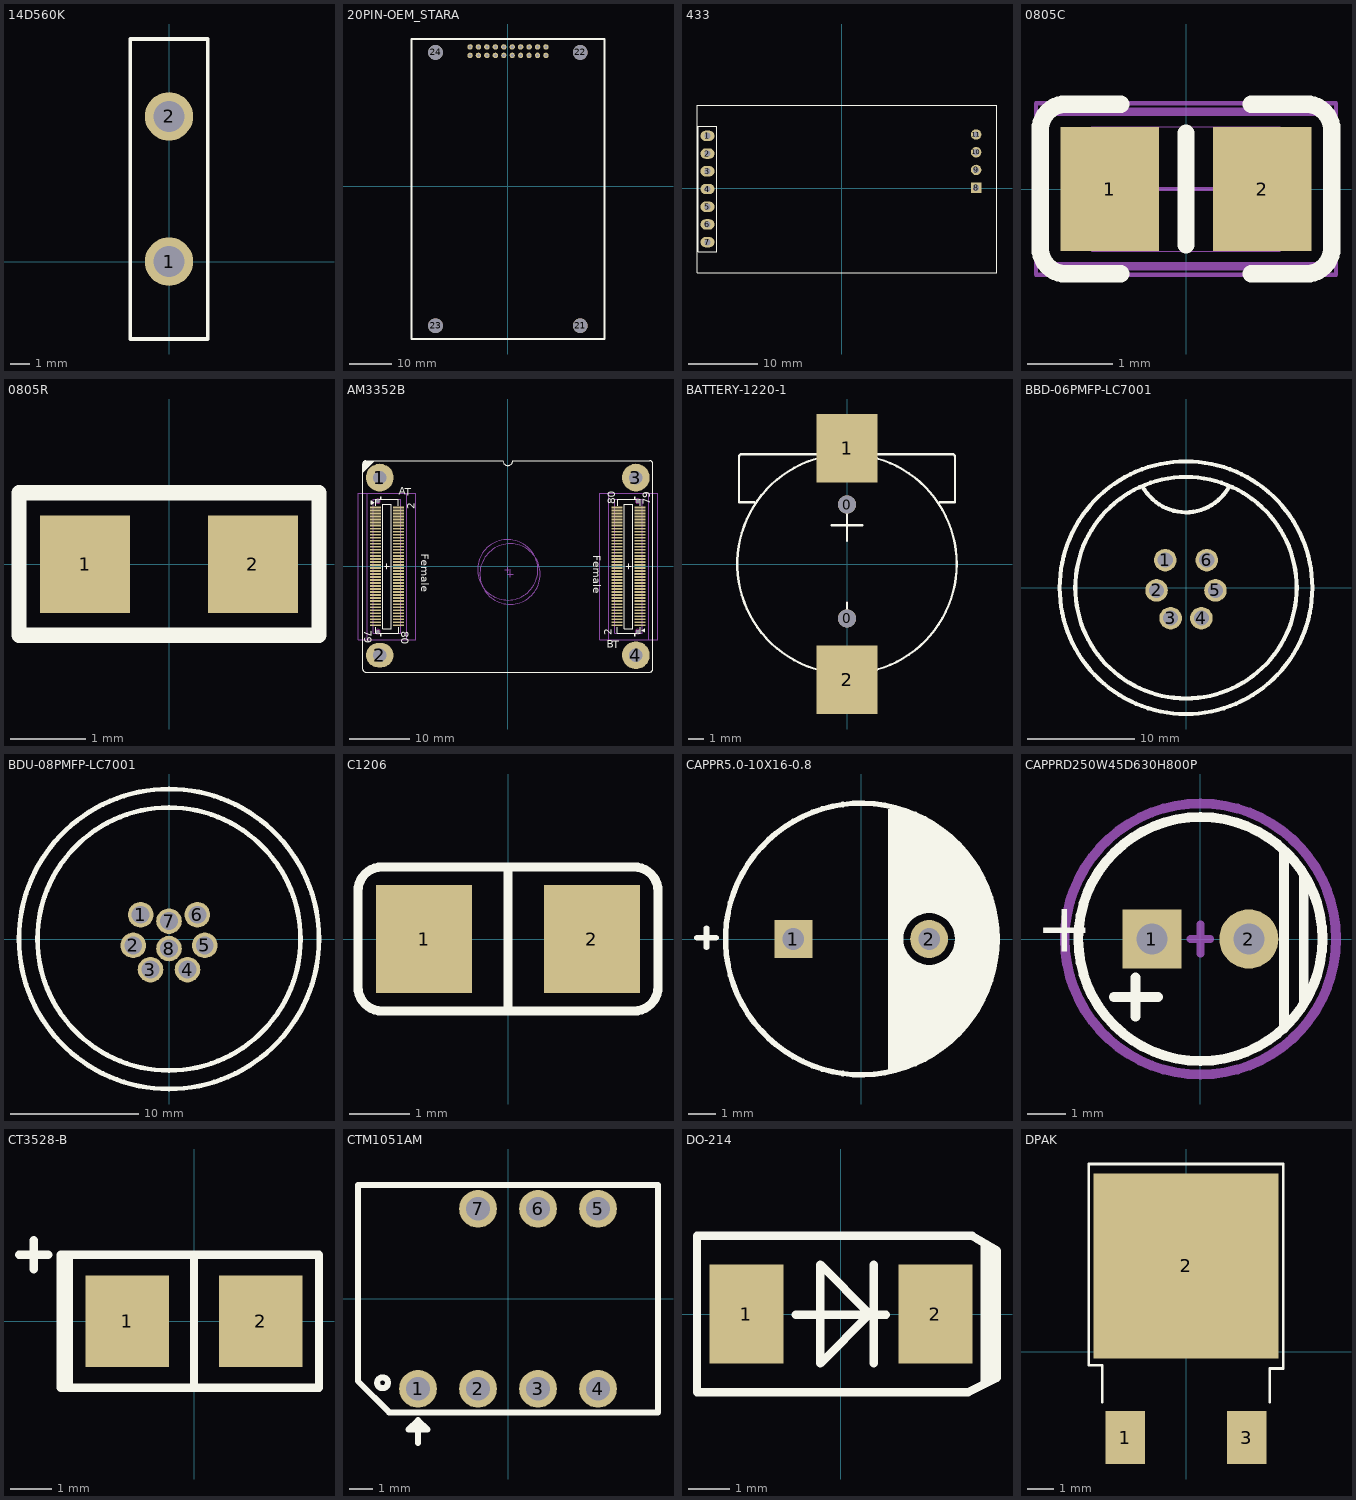
[diagram p0: the footprints below, top view; thin cyan lines are the x and y axes]
# Altium footprint library MISC82794-2.PcbLib: 41 footprints (part 1 of 3)
Each footprint in its own frame and in the unit in brackets; x right, y up, seen from the top. Pads: shape width x height; smd on the part's side, far side on the other; paste and mask are expansions set on the pad; w line width, h text height; cw(c..) or ccw(c..) is an arc to the next point about the centre after c.

## 14D560K [mm]
height 3.98
pads (2):
  round 2.5 hole 1.6: 1(0,0) 2(0,7.5)
Top Overlay:
  lines w0.2: -2,-4 -2,11.5 2,11.5 2,-4 -2,-4

## 20PIN-OEM_STARA [mm]
height 9.5
pads (24):
  round 1.3 hole 0.737: 1(-8.975,33.025) 2(-8.975,31.025) 3(-6.975,33.025) 4(-6.975,31.025) 5(-4.975,33.025) 6(-4.975,31.025) 7(-2.975,33.025) 8(-2.975,31.025) 9(-0.975,33.025) 11(1.025,33.025) 13(3.025,33.025) 15(5.025,33.025) 17(7.025,33.025) 19(9.025,33.025) 20(9.025,31.025)
  oval 1.2x1.3 hole 0.737: 10(-0.975,31.025) 12(1.025,31.025) 14(3.025,31.025) 16(5.025,31.025) 18(7.025,31.025)
  round 3.5 hole 3.5: 21(17.145,-33.025) 22(17.145,31.745) 23(-17.145,-33.025) 24(-17.145,31.745)
Top Overlay:
  lines w0.5: -22.805,-36.185 22.855,-36.185 22.855,34.915 -22.805,34.915 -22.805,-36.185

## 433 [mm]
pads (11):
  oval 2x1.5 hole 0.9: 1(-19.25,7.525) 2(-19.25,4.985) 3(-19.25,2.445) 4(-19.25,-0.095) 5(-19.25,-2.635) 6(-19.25,-5.175) 7(-19.25,-7.715)
  rect 1.5x1.5 hole 0.9: 8(19.25,0.095)
  round 1.5 hole 0.9: 9(19.25,2.635) 10(19.25,5.175) 11(19.25,7.715)
Top Overlay:
  lines w0.1: -20.75,-12.095 22.25,-12.095 22.25,11.905 -20.75,11.905 -20.75,-12.095
  lines w0.127: -20.55,-9.095 -20.55,8.905 -17.95,8.905 -17.95,-9.095 -20.55,-9.095

## 0805C [mm]
height 9.5
pads (2):
  rect 1.15x1.45 smd: 1(-0.889,0) 2(0.889,0)
Top Overlay:
  lines w0.2: 0,-0.65 0,0.65
  lines w0.203: -0.762,-0.991 -1.397,-0.991 cw(c-1.397,-0.686) -1.702,-0.686 -1.702,0.686 cw(c-1.397,0.686) -1.397,0.991 -0.762,0.991 ; 0.762,-0.991 1.397,-0.991 ccw(c1.397,-0.686) 1.702,-0.686 1.702,0.686 ccw(c1.397,0.686) 1.397,0.991 0.762,0.991
Mechanical 15:
  lines w0.1: -1.65,-0.9 -1.65,0.9 1.65,0.9 1.65,-0.9 -1.65,-0.9
  text "1" at -0.164,-0.45 h1.27
Mechanical 16:
  lines w0.001: -1.1,-0.725 -1.1,0.725 1.1,0.725 1.1,-0.725 -1.1,-0.725
  lines w0.05: -0.5,0 0.5,0 ; 0,-0.5 0,0.5 ; -1.75,-1 -1.75,1 1.75,1 1.75,-1 -1.75,-1
3D body: height 0.78, standoff 0, extent -1,-0.625 1,0.625

## 0805R [mm]
height 1.2
pads (2):
  rect 1.2x1.3 smd: 1(-1.118,0) 2(1.118,0)
Top Overlay:
  lines w0.203: -2,-0.95 -2,0.95 2,0.95 2,-0.95 -2,-0.95

## AM3352B [mm]
height 3.98
pads (172):
  round 0.6 hole 0.6 unplated mask+0.254: 0(-21.5,-10.8) 0(-21.5,-10.8) 0(-21.5,10.8) 0(-21.5,10.8) 0(21.5,-10.8) 0(21.5,-10.8) 0(21.5,10.8) 0(21.5,10.8)
  round 4.6 hole 2.2: 1(-21.2,14.7) 3(21.2,14.7) 4(21.2,-14.7)
  oval 4.6x4 hole 2.2: 2(-21.2,-14.7)
  rect 1.8x0.3 smd: A1(-21.9,9.75) A2(-18.1,9.75) A3(-21.9,9.25) A4(-18.1,9.25) A5(-21.9,8.75) A6(-18.1,8.75) A7(-21.9,8.25) A8(-18.1,8.25) A9(-21.9,7.75) A10(-18.1,7.75) A11(-21.9,7.25) A12(-18.1,7.25) A13(-21.9,6.75) A14(-18.1,6.75) A15(-21.9,6.25) A16(-18.1,6.25) A17(-21.9,5.75) A18(-18.1,5.75) A19(-21.9,5.25) A20(-18.1,5.25) A21(-21.9,4.75) A22(-18.1,4.75) A23(-21.9,4.25) A24(-18.1,4.25) A25(-21.9,3.75) A26(-18.1,3.75) A27(-21.9,3.25) A28(-18.1,3.25) A29(-21.9,2.75) A30(-18.1,2.75) A31(-21.9,2.25) A32(-18.1,2.25) A33(-21.9,1.75) A34(-18.1,1.75) A35(-21.9,1.25) A36(-18.1,1.25) A37(-21.9,0.75) A38(-18.1,0.75) A39(-21.9,0.25) A40(-18.1,0.25) A41(-21.9,-0.25) A42(-18.1,-0.25) A43(-21.9,-0.75) A44(-18.1,-0.75) A45(-21.9,-1.25) A46(-18.1,-1.25) A47(-21.9,-1.75) A48(-18.1,-1.75) A49(-21.9,-2.25) A50(-18.1,-2.25) A51(-21.9,-2.75) A52(-18.1,-2.75) A53(-21.9,-3.25) A54(-18.1,-3.25) A55(-21.9,-3.75) A56(-18.1,-3.75) A57(-21.9,-4.25) A58(-18.1,-4.25) A59(-21.9,-4.75) A60(-18.1,-4.75) A61(-21.9,-5.25) A62(-18.1,-5.25) A63(-21.9,-5.75) A64(-18.1,-5.75) A65(-21.9,-6.25) A66(-18.1,-6.25) A67(-21.9,-6.75) A68(-18.1,-6.75) A69(-21.9,-7.25) A70(-18.1,-7.25) A71(-21.9,-7.75) A72(-18.1,-7.75) A73(-21.9,-8.25) A74(-18.1,-8.25) A75(-21.9,-8.75) A76(-18.1,-8.75) A77(-21.9,-9.25) A78(-18.1,-9.25) A79(-21.9,-9.75) A80(-18.1,-9.75) B1(21.9,-9.75) B2(18.1,-9.75) B3(21.9,-9.25) B4(18.1,-9.25) B5(21.9,-8.75) B6(18.1,-8.75) B7(21.9,-8.25) B8(18.1,-8.25) B9(21.9,-7.75) B10(18.1,-7.75) B11(21.9,-7.25) B12(18.1,-7.25) B13(21.9,-6.75) B14(18.1,-6.75) B15(21.9,-6.25) B16(18.1,-6.25) B17(21.9,-5.75) B18(18.1,-5.75) B19(21.9,-5.25) B20(18.1,-5.25) B21(21.9,-4.75) B22(18.1,-4.75) B23(21.9,-4.25) B24(18.1,-4.25) B25(21.9,-3.75) B26(18.1,-3.75) B27(21.9,-3.25) B28(18.1,-3.25) B29(21.9,-2.75) B30(18.1,-2.75) B31(21.9,-2.25) B32(18.1,-2.25) B33(21.9,-1.75) B34(18.1,-1.75) B35(21.9,-1.25) B36(18.1,-1.25) B37(21.9,-0.75) B38(18.1,-0.75) B39(21.9,-0.25) B40(18.1,-0.25) B41(21.9,0.25) B42(18.1,0.25) B43(21.9,0.75) B44(18.1,0.75) B45(21.9,1.25) B46(18.1,1.25) B47(21.9,1.75) B48(18.1,1.75) B49(21.9,2.25) B50(18.1,2.25) B51(21.9,2.75) B52(18.1,2.75) B53(21.9,3.25) B54(18.1,3.25) B55(21.9,3.75) B56(18.1,3.75) B57(21.9,4.25) B58(18.1,4.25) B59(21.9,4.75) B60(18.1,4.75) B61(21.9,5.25) B62(18.1,5.25) B63(21.9,5.75) B64(18.1,5.75) B65(21.9,6.25) B66(18.1,6.25) B67(21.9,6.75) B68(18.1,6.75) B69(21.9,7.25) B70(18.1,7.25) B71(21.9,7.75) B72(18.1,7.75) B73(21.9,8.25) B74(18.1,8.25) B75(21.9,8.75) B76(18.1,8.75) B77(21.9,9.25) B78(18.1,9.25) B79(21.9,9.75) B80(18.1,9.75)
Top Overlay:
  circle w0.203: c-21.016,11.39 r0.102
  circle w0.203: c-21.016,-11.39 r0.102
  circle w0.203: c21.016,-11.39 r0.102
  circle w0.203: c21.016,11.39 r0.102
  region: -23.922,15.697 -22.195,17.424 -23.568,17.424 -23.922,17.069
  region: -22.159,10.566 -22.642,10.283 -22.642,10.85
  region: 22.159,-10.566 22.642,-10.282 22.642,-10.85
  lines w0.102: -24,-17 ccw(c-23.5,-17) -23.5,-17.5 23.5,-17.5 ccw(c23.5,-17) 24,-17 24,17 ccw(c23.5,17) 23.5,17.5 0.8,17.5 cw(c0,17.5) -0.8,17.5 -23.5,17.5 ccw(c-23.5,17) -24,17 -24,-17 ; -23.922,15.697 -23.922,16.924 cw(c-23.422,16.924) -23.422,17.424 -22.195,17.424 -23.922,15.697
  lines w0.127: -21.9,-10.084 -21.9,-11.1 -18.1,-11.1 -18.1,-10.084 ; -21.9,10.084 -21.9,11.1 -18.1,11.1 -18.1,10.084 ; 18.1,-10.084 18.1,-11.1 21.9,-11.1 21.9,-10.084 ; 18.1,10.084 18.1,11.1 21.9,11.1 21.9,10.084 ; -22.642,10.283 -22.159,10.566 -22.642,10.85 -22.642,10.283 ; -20.686,-10.3 -20.686,10.3 -19.314,10.3 -19.314,-10.3 -20.686,-10.3 ; 19.314,-10.3 20.686,-10.3 20.686,10.3 19.314,10.3 19.314,-10.3 ; 22.159,-10.566 22.642,-10.85 22.642,-10.282 22.159,-10.566
  lines w0.203: -20.4,0 -20,0 ; -20,-0.4 -20,0 ; -20,0.4 -20,0 ; -19.6,0 -20,0 ; 19.6,0 20,0 ; 20,-0.4 20,0 ; 20,0.4 20,0 ; 20.4,0 20,0
  text "T" at -15.951,11.735 h1.27
  text "80" at -17.628,-10.693 h1.27
  text "79" at -23.774,-10.566 h1.27
  text "2" at -15.443,9.423 h1.27
  text "Female" at -14.3,2.134 h1.27
  text "T" at 18.415,-13.564 h1.27
  text "80" at 17.78,10.262 h1.27
  text "79" at 23.597,10.211 h1.27
  text "2" at 17.17,-11.379 h1.27
  text "Female" at 14.122,1.829 h1.27
  text "A" at -18.059,11.836 h1.27
  text "B" at 16.358,-13.487 h1.27
Bottom Overlay:
  region: -22.083,10.566 -22.565,10.85 -22.565,10.283
  region: 22.083,-10.566 22.565,-10.85 22.565,-10.282
  region: -22.083,10.566 -22.565,10.85 -22.565,10.283
  lines w0.127: -22.565,10.283 -22.565,10.85 -22.083,10.566 -22.565,10.283 ; 22.083,-10.566 22.565,-10.85 22.565,-10.282 22.083,-10.566
Keep-Out Layer:
  circle w0.127: c-21.5,10.8 r0.38
  circle w0.127: c-21.5,10.8 r0.38
  circle w0.127: c21.5,-10.8 r0.38
  circle w0.127: c-21.5,-10.8 r0.38
  circle w0.127: c-21.5,-10.8 r0.38
  circle w0.127: c21.5,-10.8 r0.38
  circle w0.127: c21.5,10.8 r0.38
Mechanical 13:
  lines w0.152: -22.3,-11.1 -17.7,-11.1 -17.7,11.1 -22.3,11.1 -22.3,-11.1 ; 17.7,-11.1 17.7,11.1 22.3,11.1 22.3,-11.1 17.7,-11.1
Mechanical 15:
  lines w0.127: -20.432,0 -20,0 ; -20,-0.432 -20,0 ; -20,0.432 -20,0 ; -19.568,0 -20,0 ; 19.568,0 20,0 ; 20,-0.432 20,0 ; 20,0.432 20,0 ; 20.432,0 20,0
  lines w0.152: -23.3,-12.1 -23.3,12.1 ; -16.7,-12.1 -16.7,12.1 ; 16.7,-12.1 16.7,12.1 ; 23.3,-12.1 23.3,12.1 ; -24.8,-12.1 -24.8,12.1 -15.2,12.1 -15.2,-12.1 -24.8,-12.1 ; 15.2,-12.1 24.8,-12.1 24.8,12.1 15.2,12.1 15.2,-12.1
  text "0.6mm机械孔径公差要求为（0,+0.05）mm" at -19.67,-8.306 h1.27
  text "元件禁布区" at -15.453,-3.353 h1.27
  text "元件禁布区" at -23.531,-3.353 h1.27
  text "0.6mm机械孔径公差要求为（0,+0.05）mm" at 19.67,8.306 h1.27
  text "元件禁布区" at 15.453,3.353 h1.27
  text "元件禁布区" at 23.531,3.353 h1.27
Mechanical 16:
  circle w0.001: c-0.017,-0.564 r5
  circle w0.001: c0.378,-1.264 r5
  lines w0.05: -0.517,-0.564 0.483,-0.564 ; -0.122,-1.264 0.878,-1.264 ; -0.017,-1.064 -0.017,-0.064 ; 0.378,-1.764 0.378,-0.764

## BATTERY-1220-1 [mm]
height 9.5
pads (4):
  round 1.2 hole 1.2: 0(0,-3.581) 0(0,3.912)
  rect 4x4.5 smd: 1(0,7.62) 2(0,-7.62)
Top Overlay:
  circle w0.152: c0,0 r7.22
  lines w0.152: -6.096,4.064 -7.112,4.064 -7.112,7.112 -7.004,7.22 0,7.22 7.004,7.22 7.112,7.112 7.112,4.064 6.096,4.064 ; -1.016,2.54 1.016,2.54 ; 0,-4.064 0,-2.54 ; 0,1.524 0,3.556

## BBD-06PMFP-LC7001 [mm]
pads (6):
  round 2.1 hole 1.4: 1(-1.93,2.56) 2(-2.74,-0.25) 3(-1.43,-2.84) 4(1.43,-2.84) 5(2.74,-0.25) 6(1.93,2.56)
Top Overlay:
  circle w0.381: c0,0 r11.75
  circle w0.381: c0,0 r10.3
  lines w0.381: -4.005,9.36 ccw(c-0.009,11.584) 3.937,9.271

## BDU-08PMFP-LC7001 [mm]
pads (8):
  round 2 hole 1.4: 1(-2.22,1.9) 2(-2.8,-0.5) 3(-1.45,-2.4) 4(1.45,-2.4) 5(2.8,-0.5) 6(2.22,1.9) 7(0,1.4) 8(0,-0.75)
Top Overlay:
  circle w0.381: c0,0 r11.75
  circle w0.381: c0,0 r10.3

## C1206 [mm]
pads (2):
  rect 1.6x1.8 smd: 1(-1.4,0) 2(1.4,0)
Top Overlay:
  lines w0.152: 0,-1.2 0,1.2 ; -2.5,-0.8 ccw(c-2.1,-0.8) -2.1,-1.2 2.1,-1.2 ccw(c2.1,-0.8) 2.5,-0.8 2.5,0.8 ccw(c2.1,0.8) 2.1,1.2 -2.1,1.2 ccw(c-2.1,0.8) -2.5,0.8 -2.5,-0.8
3D body: height 0.61, standoff 0, extent -1.524,-0.818 1.524,0.711

## CAPPR5.0-10X16-0.8 [mm]
height 3.98
pads (2):
  rect 1.4x1.4 hole 0.8: 1(-2.5,0)
  round 1.4 hole 0.8: 2(2.5,0)
Top Overlay:
  circle w0.203: c0,0 r5
  circle w0.5: c2.5,0 r1.2
  rectangle: 4.511,-1.09 4.911,1.41
  rectangle: 4.1,-1.8 4.6,2.2
  rectangle: 3.7,-2.6 4.2,2.8
  rectangle: 1.5,-4.2 2.8,-3.3
  rectangle: 1.5,-3.5 3.5,-1
  rectangle: 3.5,-3.2 3.8,3.3
  rectangle: 2.7,1 3.5,3.6
  rectangle: 1.45,1 2.8,4.2
  rectangle: 1.3,-4.7 1.5,4.8
  rectangle: 0.989,-4.81 1.389,4.79
  lines w0.203: -6.05,0.05 -5.7,0.05 ; -5.7,-0.3 -5.7,0.05 ; -5.7,0.4 -5.7,0.05 ; -5.35,0.05 -5.7,0.05
  lines w1: 1.514,-4.238 ccw(c0,0) 1.569,4.217
3D body: height 15.68, standoff -2.45, extent -5.1,-5.1 4.9,4.9

## CAPPRD250W45D630H800P [mm] "6.5mm"
height 8
pads (2):
  rect 1.524x1.524 hole 0.8: 1(-1.25,0)
  round 1.524 hole 0.8: 2(1.25,0)
Top Overlay:
  circle w0.254: c0,0 r3.15
  lines w0.254: -2.235,-1.499 -1.092,-1.499 ; -1.676,-2.007 -1.676,-0.991 ; 2.159,-2.311 2.159,2.261 ; 2.667,-1.676 2.667,1.626
  text "+" at -4.242,-0.33 h1.27
Mechanical 15:
  circle w0.254: c0,0 r3.5
  lines w0.203: -0.254,0 0,0 ; 0,-0.381 0,0 ; 0,0.381 0,0 ; 0.254,0 0,0
3D body: height 11.5, standoff -18.5, extent -3.15,-3.15 3.15,3.15

## CT3528-B [mm]
pads (2):
  rect 2x2.2 smd: 1(-1.6,0) 2(1.6,0)
Top Overlay:
  rectangle: -3.2,-1.5 -2.9,1.5
  lines w0.203: -4.2,1.6 -3.85,1.6 ; -3.85,1.25 -3.85,1.6 ; -3.85,1.95 -3.85,1.6 ; -3.5,1.6 -3.85,1.6 ; 0,-1.6 0,1.5 ; -3.2,-1.6 3,-1.6 3,1.6 -3.2,1.6 -3.2,-1.6
3D body: height 1.9, standoff 0, extent -1.75,-1.4 1.75,1.4

## CTM1051AM [mm] "7.7mm"
pads (7):
  round 1.6 hole 1: 1(-3.81,-3.81) 2(-1.27,-3.81) 3(1.27,-3.81) 4(3.81,-3.81) 5(3.81,3.81) 6(1.27,3.81) 7(-1.27,3.81)
Top Overlay:
  circle w0.254: c-5.31,-3.556 r0.23
  lines w0.254: -3.81,-6.096 -3.81,-5.131 ; -3.81,-5.131 -4.216,-5.537 -3.404,-5.537 -3.81,-5.131 ; -6.35,-3.489 -5.029,-4.81 6.35,-4.81 6.35,4.81 -6.35,4.81 -6.35,-3.489

## DO-214 [mm]
height 9.5
pads (2):
  rect 1.8x2.4 smd: 1(-2.3,0) 2(2.3,0)
Top Overlay:
  lines w0.203: -1.1,-0.02 1.1,-0.02 ; 0.8,-1.2 0.8,1.2 ; 3.5,-1.7 3.5,1.7 ; 3.7,-1.5 3.7,1.6 ; -3.5,-1.9 -3.5,1.9 3.2,1.9 3.8,1.54 3.8,-1.55 3.1,-1.9 -3.5,-1.9 ; -0.5,-1.2 -0.5,1.2 0.7,0 -0.5,-1.2

## DPAK [mm]
pads (3):
  rect 1.5x2 smd: 1(-2.3,-3.25) 3(2.3,-3.25)
  rect 7x7 smd: 2(0,3.25)
Top Overlay:
  lines w0.1: -3.175,-1.905 -3.175,-0.508 -3.683,-0.508 -3.683,6.858 -3.683,7.112 3.683,7.112 3.683,6.858 3.683,-0.635 3.175,-0.635 3.175,-1.905